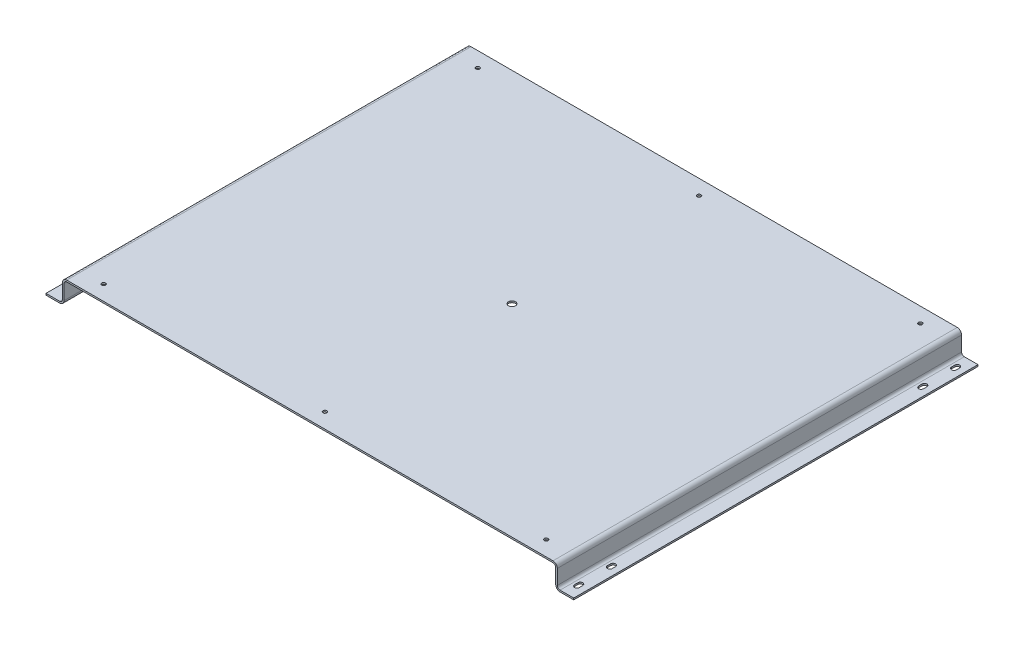
SolidWorks part; units mm, degrees
material "1023 碳钢板 (SS)"
ref_plane "前视基准面" through (0, 0, 0) normal (0, 0, 1) x (1, 0, 0)
ref_plane "上视基准面" through (0, 0, 0) normal (0, 1, 0) x (1, 0, 0)
ref_plane "右视基准面" through (0, 0, 0) normal (1, 0, 0) x (0, 0, -1)
sketch "草图1" plane through (0, 0, 0) normal (0, 0, 1) x (1, 0, 0)
  line L0 (0, 0) -> (25, 0)
  line L1 (33, 8) -> (33, 35)
  line L2 (38, 40) -> (928, 40)
  line L3 (933, 35) -> (933, 8)
  line L4 (941, 0) -> (966, 0)
  line L5 (0, 3) -> (25, 3)
  line L6 (30, 8) -> (30, 35)
  line L7 (38, 43) -> (928, 43)
  line L8 (936, 35) -> (936, 8)
  line L9 (941, 3) -> (966, 3)
  line L10 (966, 3) -> (966, 0)
  line L11 (0, 3) -> (0, 0)
  line L12 (0, 3) -> (30, 3) construction
  line L13 (30, 3) -> (30, 35) construction
  line L14 (936, 35) -> (936, 3) construction
  line L15 (936, 3) -> (966, 3) construction
  line L16 (0, 0) -> (33, 0) construction
  line L17 (33, 0) -> (33, 35) construction
  line L18 (933, 35) -> (933, 0) construction
  line L19 (933, 0) -> (966, 0) construction
  arc A0 (933, 35) -> (928, 40) centre (928, 35) ccw
  arc A1 (33, 35) -> (38, 40) centre (38, 35) cw
  arc A2 (30, 35) -> (38, 43) centre (38, 35) cw
  arc A3 (936, 35) -> (928, 43) centre (928, 35) ccw
  arc A4 (25, 3) -> (30, 8) centre (25, 8) ccw
  arc A5 (936, 8) -> (941, 3) centre (941, 8) ccw
  arc A6 (25, 0) -> (33, 8) centre (25, 8) ccw
  arc A7 (933, 8) -> (941, 0) centre (941, 8) ccw
  point P9 (933, 40)
  point P12 (33, 40)
  point P32 (33, 0)
  point P36 (933, 0)
  dimension "D5" = 5
  dimension "D7" = 5
  dimension "D8" = 5
  dimension "D9" = 8
  dimension "D1" = 33
  dimension "D2" = 33
  dimension "D3" = 900
  dimension "D4" = 40
  dimension "D6" = 3
extrude "凸台-拉伸1" add sketch "草图1" along normal blind 740 contours L11 L0 A6 L1 A1 L2 A0 L3 A7 L4 L10 L9 A5 L8 A3 L7 A2 L6 A4 L5
sketch "草图2" plane through (0, 43, 0) normal (0, 1, 0) x (1, 0, 0)
  line L0 (38, -370) -> (496.82, -370) construction
  line L1 (38, -740) -> (38, 0) construction
  line L2 (38, -740) -> (928, -740) construction
  line L3 (25, -740) -> (25, 0) construction
  circle A0 centre (78, -27.5) radius 3.5
  circle A1 centre (483, -27.5) radius 3.5
  circle A2 centre (888, -27.5) radius 3.5
  circle A3 centre (78, -712.5) radius 3.5
  circle A4 centre (888, -712.5) radius 3.5
  circle A5 centre (483, -712.5) radius 3.5
  dimension "D6" = 7
  dimension "D1" = 685
  dimension "D2" = 27.5
  dimension "D3" = 53
  dimension "D4" = 405
  dimension "D5" = 405
extrude "切除-拉伸1" cut sketch "草图2" against normal blind 740
sketch "草图3" plane through (0, 3, 0) normal (0, 1, 0) x (1, 0, 0)
  line L0 (16, -22) -> (16, -28) construction
  line L1 (20.5, -22) -> (20.5, -28)
  line L2 (11.5, -22) -> (11.5, -28)
  line L3 (0, -740) -> (0, 0) construction
  line L4 (0, 0) -> (25, 0) construction
  line L5 (16, -82) -> (16, -88) construction
  line L8 (20.5, -82) -> (20.5, -88)
  line L9 (11.5, -82) -> (11.5, -88)
  line L10 (0, -370) -> (179.3413, -370) construction
  line L11 (483, 0) -> (483, -104.5933) construction
  line L12 (38, 0) -> (928, 0) construction
  line L13 (950, -82) -> (950, -88) construction
  line L14 (945.5, -82) -> (945.5, -88)
  line L15 (954.5, -82) -> (954.5, -88)
  line L16 (950, -22) -> (950, -28) construction
  line L17 (945.5, -22) -> (945.5, -28)
  line L18 (954.5, -22) -> (954.5, -28)
  line L19 (950, -658) -> (950, -652) construction
  line L20 (945.5, -658) -> (945.5, -652)
  line L21 (954.5, -658) -> (954.5, -652)
  line L22 (950, -718) -> (950, -712) construction
  line L23 (945.5, -718) -> (945.5, -712)
  line L24 (954.5, -718) -> (954.5, -712)
  line L25 (16, -658) -> (16, -652) construction
  line L26 (20.5, -658) -> (20.5, -652)
  line L27 (11.5, -658) -> (11.5, -652)
  line L28 (16, -718) -> (16, -712) construction
  line L29 (20.5, -718) -> (20.5, -712)
  line L30 (11.5, -718) -> (11.5, -712)
  arc A0 (20.5, -22) -> (11.5, -22) centre (16, -22) ccw
  arc A1 (11.5, -28) -> (20.5, -28) centre (16, -28) ccw
  arc A4 (20.5, -82) -> (11.5, -82) centre (16, -82) ccw
  arc A5 (11.5, -88) -> (20.5, -88) centre (16, -88) ccw
  arc A6 (945.5, -82) -> (954.5, -82) centre (950, -82) cw
  arc A7 (954.5, -88) -> (945.5, -88) centre (950, -88) cw
  arc A8 (945.5, -22) -> (954.5, -22) centre (950, -22) cw
  arc A9 (954.5, -28) -> (945.5, -28) centre (950, -28) cw
  arc A10 (945.5, -658) -> (954.5, -658) centre (950, -658) ccw
  arc A11 (954.5, -652) -> (945.5, -652) centre (950, -652) ccw
  arc A12 (945.5, -718) -> (954.5, -718) centre (950, -718) ccw
  arc A13 (954.5, -712) -> (945.5, -712) centre (950, -712) ccw
  arc A14 (20.5, -658) -> (11.5, -658) centre (16, -658) cw
  arc A15 (11.5, -652) -> (20.5, -652) centre (16, -652) cw
  arc A16 (20.5, -718) -> (11.5, -718) centre (16, -718) cw
  arc A17 (11.5, -712) -> (20.5, -712) centre (16, -712) cw
  point P2 (16, -25)
  point P7 (16, -85)
  point P26 (950, -85)
  point P33 (950, -25)
  point P40 (950, -655)
  point P47 (950, -715)
  point P54 (16, -655)
  point P61 (16, -715)
  dimension "D1" = 4.5
  dimension "D3" = 16
  dimension "D6" = 4.5
  dimension "D8" = 60
  dimension "D2" = 6
  dimension "D4" = 22
  dimension "D5" = 6
  dimension "D7" = 16
extrude "切除-拉伸2" cut sketch "草图3" against normal blind 740
sketch "草图4" plane through (0, 43, 0) normal (0, 1, 0) x (1, 0, 0)
  line L0 (928, -740) -> (928, 0) construction
  circle A0 centre (483, -370) radius 6.5
  point P2 (0, 0)
  point P5 (928, -370)
  dimension "D1" = 13
extrude "切除-拉伸3" cut sketch "草图4" against normal blind 10
